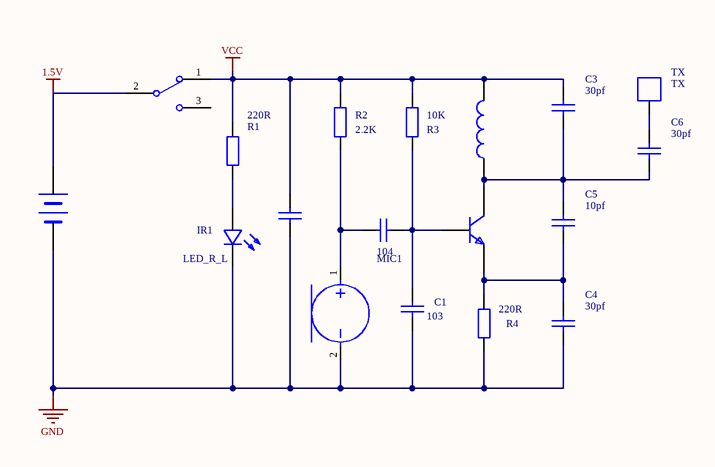
[diagram p0: MISC51881-3.schdoc]
# Altium project MISC51881-2.PrjPcb
1 sheet, 18 parts. Net scope: global (net labels, ports and power ports of the same name join across sheets).
Board file: MISC51881.pcbdoc

## Sheet MISC51881-3.schdoc
size 297 x 209 mm; Version: V1.0; @Project Name: MISC51881; @Update Date: 2026-03-18; @Create Date: 2026-03-18; @Board Name: MISC51881; @Create Time: 14:12:05; @Page Count: 1; @Page No: 1; @Schematic Name: MISC51881; @Update Time: 14:12:05; Size: A4

### Parts
BT1  BATTERY  [Bat_Box_01]  (value not drawn)
C1  103  [CC 1.8*3.6]
C2  104  [CC 2.2*5]
C3  30pf  [CC 1.8*3.6]
C4  30pf  [CC 1.8*3.6]
C5  10pf  [CC 1.8*3.6]
C6  30pf  [CC 1.8*3.6]
C7  104  [CC 2.2*5]  (value not drawn)
IR1  LED_R_L  [LED-TH_BD5.0-P2.54-FD]
L1  4T  [IND_5x5]  (value not drawn)
MIC1  MIC  [MIC-TH_BD6.0-P1.90-D0.4-L-FD_GMI6050P-2CXXDB]  (value not drawn)
Q1  9018  [TANS]  (value not drawn)
R1  Res  [AXIAL0.4-1/4W]  (value not drawn)
R2  Res  [AXIAL0.4-1/4W]  (value not drawn)
R3  Res  [AXIAL0.4-1/4W]  (value not drawn)
R4  Res  [AXIAL0.4-1/4W]  (value not drawn)
S1  MTS-10x  [SW-TH_KH-SS12D01-G3-5.0]  (value not drawn)
TX  TX  [TX]

### Nets
1.5V: BT1.1(+) S1.2
GND: BT1.2(-) C1.1 C4.1 C7.1 IR1.2(C) MIC1.2 R4.1
VCC: C3.2 C7.2 L1.1 R1.2 R2.2 R3.2 S1.1
NetC1_2: C1.2 C2.2 Q1.2(B) R3.1
NetC2_1: C2.1 MIC1.1 R2.1
NetC3_1: C3.1 C5.2 C6.1 L1.2 Q1.3(C)
NetC4_2: C4.2 C5.1 Q1.1(E) R4.2
NetC6_2: C6.2 TX.1
NetIR1_1: IR1.1(A) R1.1

Not connected (* = marked no-connect by the designer): S1 3

### Notes on the sheet
- 2026-03-18
- Schematic
- Board
- Sheet
- P1
- Drawn by
- Reviewed
- Revision
- Size
- A4
- page 1 Total 1

### Library data of the parts
BT1 = BATTERY: AddInBom: yes; Symbol: BATTERY; Device: BATTERY; ConvertToPcb: yes; FootprintName: Bat_Box_01
C1 = 103: AddInBom: yes; Symbol: 103; Device: 103; ConvertToPcb: yes; Published: 8-Jun-2000; LatestRevisionDate: 17-Jul-2002; LatestRevisionNote: Re-released for DXP Platform.; PackageReference: RAD-0.3; FootprintName: CC 1.8*3.6; Publisher: Altium Limited
C2 C7 = 104: AddInBom: yes; Symbol: 104; Device: 104; ConvertToPcb: yes; Published: 8-Jun-2000; LatestRevisionDate: 17-Jul-2002; LatestRevisionNote: Re-released for DXP Platform.; PackageReference: RAD-0.3; FootprintName: CC 2.2*5; Publisher: Altium Limited
C3 C4 C6 = 30pf: AddInBom: yes; Symbol: 30pf; Device: 30pf; ConvertToPcb: yes; Published: 8-Jun-2000; LatestRevisionDate: 17-Jul-2002; LatestRevisionNote: Re-released for DXP Platform.; PackageReference: RAD-0.3; FootprintName: CC 1.8*3.6; Publisher: Altium Limited
C5 = 10pf: AddInBom: yes; Symbol: 10pf; Device: 10pf; ConvertToPcb: yes; Published: 8-Jun-2000; LatestRevisionDate: 17-Jul-2002; LatestRevisionNote: Re-released for DXP Platform.; PackageReference: RAD-0.3; FootprintName: CC 1.8*3.6; Publisher: Altium Limited
IR1 = LED_R_G: Manufacturer: VISHAY(威世); ManufacturerPart: TSAL6200; AddInBom: yes; ModelId: d69ce262ecf3444980b2005e7e1c2e8d; Symbol: LED_R_G; Device: LED_R_G; Supplier: LCSC; SupplierPart: C55528; JLCPCB Part Class: Extended library; ConvertToPcb: yes; FootprintName: LED-TH_BD5.0-P2.54-FD; ModelName: LED-TH_BD5.0-P2.54-FD
L1 = L: AddInBom: yes; Symbol: L; Device: L; ConvertToPcb: yes; FootprintName: IND_5x5
MIC1 = MIC: Manufacturer: INGHAi(赢海); ManufacturerPart: GMI9750UP-2C40DB; AddInBom: yes; Origin Footprint 2: MIC-TH_BD9.7-P2.50-D0.8-L-FD - duplicate; ModelId: 13bff40b06b543799f1cf39aeb3f973a; Symbol: MIC; Device: MIC; ConvertToPcb: yes; LCSC Part Name: GMI9750UP-2C40DB; SupplierPart: C530221; Supplier Footprint: -; JLCPCB Part Class: Extended library; Datasheet: https://atta.szlcsc.com/upload/public/pdf/source/20231017/7730F5E17633AEF7C001E490CA532738.pdf; Supplier: LCSC; FootprintName: MIC-TH_BD6.0-P1.90-D0.4-L-FD_GMI6050P-2CXXDB; ModelName: MIC-TH_BD6.0-P1.90-D0.4-L-FD_GMI6050P-2CXXDB
Q1 = 9018: AddInBom: yes; Symbol: 9018; Device: 9018; ConvertToPcb: yes; Published: 8-Jun-2000; LatestRevisionDate: 15-Jan-2003; LatestRevisionNote: PCB Footprint 'BCY-W3/D4.7' replaced; DatasheetDocument: 1997; PackageDocument: Sep-1998; PackageReference: TO-92A; Code_JEDEC: TO-92A; ComponentLink1Description: Manufacturer Link; ComponentLink2Description: Datasheet; ComponentLink2URL: http://www.fairchildsemi.com/ds/2N%2F2N3904.pdf; FootprintName: TANS; Publisher: Altium Limited
R1 R4 = 220R: AddInBom: yes; Value: 220R; Symbol: 220R; Device: 220R; ConvertToPcb: yes; Published: 8-Jun-2000; LatestRevisionDate: 17-Jul-2002; LatestRevisionNote: Re-released for DXP Platform.; PackageReference: AXIAL-0.4; FootprintName: AXIAL0.4-1/4W; Publisher: Altium Limited
R2 = 2.2K: AddInBom: yes; Value: 2.2K; Symbol: 2.2K; Device: 2.2K; ConvertToPcb: yes; Published: 8-Jun-2000; LatestRevisionDate: 17-Jul-2002; LatestRevisionNote: Re-released for DXP Platform.; PackageReference: AXIAL-0.4; FootprintName: AXIAL0.4-1/4W; Publisher: Altium Limited
R3 = 10K: AddInBom: yes; Value: 10K; Symbol: 10K; Device: 10K; ConvertToPcb: yes; Published: 8-Jun-2000; LatestRevisionDate: 17-Jul-2002; LatestRevisionNote: Re-released for DXP Platform.; PackageReference: AXIAL-0.4; FootprintName: AXIAL0.4-1/4W; Publisher: Altium Limited
S1 = MTS-10x: AddInBom: yes; BOM名称: MTS10x series 3-pin toggle switch; ModelId: 26d5331bbd27478083cc9b7d4df92690; Symbol: MTS-10x; Device: MTS-10x; ConvertToPcb: yes; FootprintName: SW-TH_KH-SS12D01-G3-5.0; ModelName: SW-TH_KH-SS12D01-G3-5.0
TX = TX: AddInBom: yes; Symbol: TX; Device: TX; ConvertToPcb: yes; FootprintName: TX